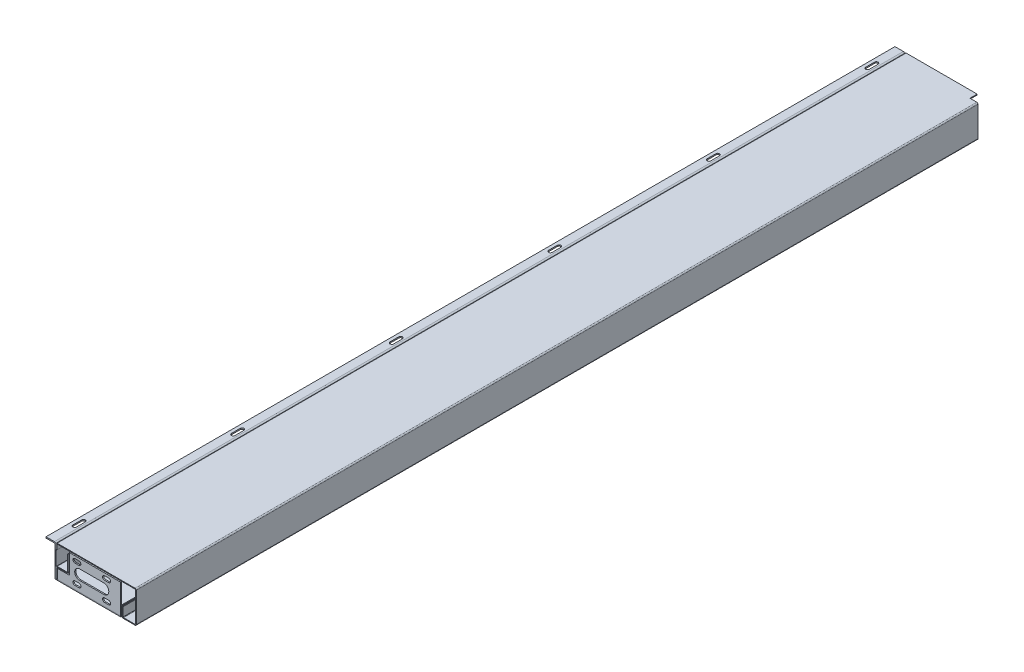
from build123d import *

# Parameters (mm, degrees)
EXTRUDE_1_DEPTH             = 1058
EXTRUDE_2_DEPTH             = 1058
EXTRUDE_2_2_DEPTH           = 1058
EXTRUDE_3_DEPTH             = 3
FILLET_1_R                  = 4
FILLET_2_R                  = 1
FILLET_3_R                  = 1
FILLET_4_R                  = 1
FILLET_5_R                  = 3
FILLET_6_R                  = 3
CUT_EXTRUDE_1_DEPTH         = 2127.935824138
CUT_EXTRUDE_3490_DEPTH      = 3
CUT_EXTRUDE_3711_DEPTH      = 1080.705515407
CUT_EXTRUDE_3711_DEPTH_BACK = 1080.705515407
SKETCH_6_W                  = 20
SKETCH_6_H                  = 18


with BuildPart() as part:
    # 草图1 → 凸台-拉伸1 (new, symmetric)
    with BuildSketch(Plane.XY):
        Polygon((-25, 0), (0, 0), (0, -80), (-3, -80), (-3, -3), (-25, -3), align=None)
    extrude(amount=EXTRUDE_1_DEPTH, both=True)

    # 圆角1
    fillet_1_edges = [part.edges().sort_by_distance(p)[0] for p in [
        (0, 0, 0),
    ]]
    fillet(fillet_1_edges, radius=FILLET_1_R)

    # 圆角2
    fillet_2_edges = [part.edges().sort_by_distance(p)[0] for p in [
        (-3, -3, 0),
    ]]
    fillet(fillet_2_edges, radius=FILLET_2_R)

    # 草图7 → Cut-Extrude 3490 (cut)
    with BuildSketch(Plane(origin=(0, 0, 0), x_dir=(1, 0, 0), z_dir=(0, 1, 0))):
        with BuildLine():
            Line((-17, 977), (-17, 999))
            ThreePointArc((-17, 999), (-12.5, 1003.5), (-8, 999))
            Line((-8, 999), (-8, 977))
            ThreePointArc((-8, 977), (-12.5, 972.5), (-17, 977))
        make_face()
        with BuildLine():
            Line((-17, 581.8), (-17, 603.8))
            ThreePointArc((-17, 603.8), (-12.5, 608.3), (-8, 603.8))
            Line((-8, 603.8), (-8, 581.8))
            ThreePointArc((-8, 581.8), (-12.5, 577.3), (-17, 581.8))
        make_face()
        with BuildLine():
            Line((-17, 186.6), (-17, 208.6))
            ThreePointArc((-17, 208.6), (-12.5, 213.1), (-8, 208.6))
            Line((-8, 208.6), (-8, 186.6))
            ThreePointArc((-8, 186.6), (-12.5, 182.1), (-17, 186.6))
        make_face()
        with BuildLine():
            Line((-17, -208.6), (-17, -186.6))
            ThreePointArc((-17, -186.6), (-12.5, -182.1), (-8, -186.6))
            Line((-8, -186.6), (-8, -208.6))
            ThreePointArc((-8, -208.6), (-12.5, -213.1), (-17, -208.6))
        make_face()
        with BuildLine():
            Line((-17, -603.8), (-17, -581.8))
            ThreePointArc((-17, -581.8), (-12.5, -577.3), (-8, -581.8))
            Line((-8, -581.8), (-8, -603.8))
            ThreePointArc((-8, -603.8), (-12.5, -608.3), (-17, -603.8))
        make_face()
        with BuildLine():
            Line((-17, -999), (-17, -977))
            ThreePointArc((-17, -977), (-12.5, -972.5), (-8, -977))
            Line((-8, -977), (-8, -999))
            ThreePointArc((-8, -999), (-12.5, -1003.5), (-17, -999))
        make_face()
    extrude(amount=-CUT_EXTRUDE_3490_DEPTH, mode=Mode.SUBTRACT)


with BuildPart() as body_2:
    # 草图2 → 凸台-拉伸2 (new, symmetric)
    with BuildSketch(Plane.XY):
        Polygon((0, 0), (0, -15), (2, -15), (2, -2), (198, -2), (198, -78), (167, -78), (167, -55), (165, -55), (165, -80), (200, -80), (200, 0), align=None)
    extrude(amount=EXTRUDE_2_DEPTH, both=True)

    # 圆角3
    fillet_3_edges = [body_2.edges().sort_by_distance(p)[0] for p in [
        (167, -78, 0),
        (198, -78, 0),
        (198, -2, 0),
        (2, -2, 0),
    ]]
    fillet(fillet_3_edges, radius=FILLET_3_R)

    # 圆角5
    fillet_5_edges = [body_2.edges().sort_by_distance(p)[0] for p in [
        (200, 0, 0),
        (200, -80, 0),
        (165, -80, 0),
        (0, 0, 0),
    ]]
    fillet(fillet_5_edges, radius=FILLET_5_R)

    # 草图6 → Cut-Extrude 3711 (cut, two sides: drawn at the far end of the back side and taken through both)
    with BuildSketch(Plane(origin=(0, 0, 0), x_dir=(1, 0, 0), z_dir=(0, 1, 0)).offset(-CUT_EXTRUDE_3711_DEPTH_BACK)):
        with Locations((190, 1049)):
            Rectangle(SKETCH_6_W, SKETCH_6_H)
    extrude(amount=CUT_EXTRUDE_3711_DEPTH + CUT_EXTRUDE_3711_DEPTH_BACK, mode=Mode.SUBTRACT)


with BuildPart() as body_3:
    # 草图2 → Extrude 2 2 (new, symmetric)
    with BuildSketch(Plane.XY):
        Polygon((0, -50), (0, -80), (163.5, -80), (163.5, -55), (161.5, -55), (161.5, -78), (2, -78), (2, -52), (30, -52), (30, -11), (28, -11), (28, -50), align=None)
    extrude(amount=EXTRUDE_2_2_DEPTH, both=True)

    # 圆角4
    fillet_4_edges = [body_3.edges().sort_by_distance(p)[0] for p in [
        (28, -50, 0),
        (2, -52, 0),
        (2, -78, 0),
        (161.5, -78, 0),
    ]]
    fillet(fillet_4_edges, radius=FILLET_4_R)

    # 圆角6
    fillet_6_edges = [body_3.edges().sort_by_distance(p)[0] for p in [
        (30, -52, 0),
        (163.5, -80, 0),
        (0, -80, 0),
        (0, -50, 0),
    ]]
    fillet(fillet_6_edges, radius=FILLET_6_R)


with BuildPart() as body_4:
    # 草图3 → 凸台-拉伸3 (new body)
    with BuildSketch(Plane.XY.offset(1058)):
        Polygon((160.5, -78), (160.5, -5), (33, -5), (33, -54), (4, -54), (4, -78), align=None)
    extrude(amount=-EXTRUDE_3_DEPTH)

    # 草图5 → 切除-拉伸1 (cut, through all)
    with BuildSketch(Plane.XY.offset(1058)):
        with BuildLine():
            Line((47, -11), (57, -11))
            ThreePointArc((57, -11), (62, -16), (57, -21))
            Line((57, -21), (47, -21))
            ThreePointArc((47, -21), (42, -16), (47, -11))
        make_face()
        with BuildLine():
            Line((47, -69), (57, -69))
            ThreePointArc((57, -69), (62, -64), (57, -59))
            Line((57, -59), (47, -59))
            ThreePointArc((47, -59), (42, -64), (47, -69))
        make_face()
        with BuildLine():
            Line((121, -11), (131, -11))
            ThreePointArc((131, -11), (136, -16), (131, -21))
            Line((131, -21), (121, -21))
            ThreePointArc((121, -21), (116, -16), (121, -11))
        make_face()
        with BuildLine():
            Line((121, -69), (131, -69))
            ThreePointArc((131, -69), (136, -64), (131, -59))
            Line((131, -59), (121, -59))
            ThreePointArc((121, -59), (116, -64), (121, -69))
        make_face()
        with BuildLine():
            Line((119, -52.5), (59, -52.5))
            ThreePointArc((59, -52.5), (46.5, -40), (59, -27.5))
            Line((59, -27.5), (119, -27.5))
            ThreePointArc((119, -27.5), (131.5, -40), (119, -52.5))
        make_face()
    extrude(amount=-CUT_EXTRUDE_1_DEPTH, mode=Mode.SUBTRACT)


with BuildPart() as body_5:
    # 镜向1: mirrored copy
    add(body_4.part.mirror(Plane.XY))


solid = Compound([part.part, body_2.part, body_3.part, body_4.part, body_5.part])
